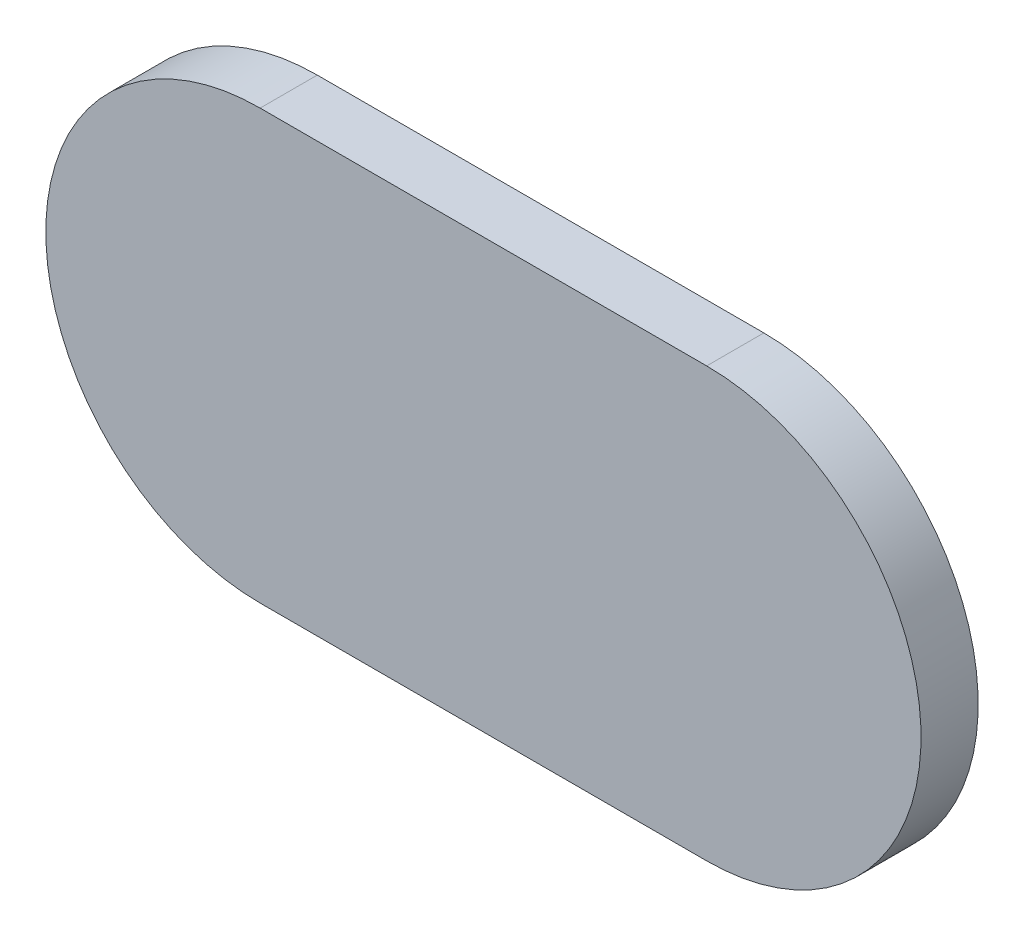
from build123d import *

# Parameters (mm, degrees)
EXTRUDE_1_DEPTH = 16


with BuildPart() as part:
    # 草图1 → 凸台-拉伸1 (new body)
    with BuildSketch(Plane.XY):
        with BuildLine():
            Line((-62.5, 60), (62.5, 60))
            ThreePointArc((62.5, 60), (122.5, 0), (62.5, -60))
            Line((62.5, -60), (-62.5, -60))
            ThreePointArc((-62.5, -60), (-122.5, 0), (-62.5, 60))
        make_face()
    extrude(amount=EXTRUDE_1_DEPTH)


solid = part.part
